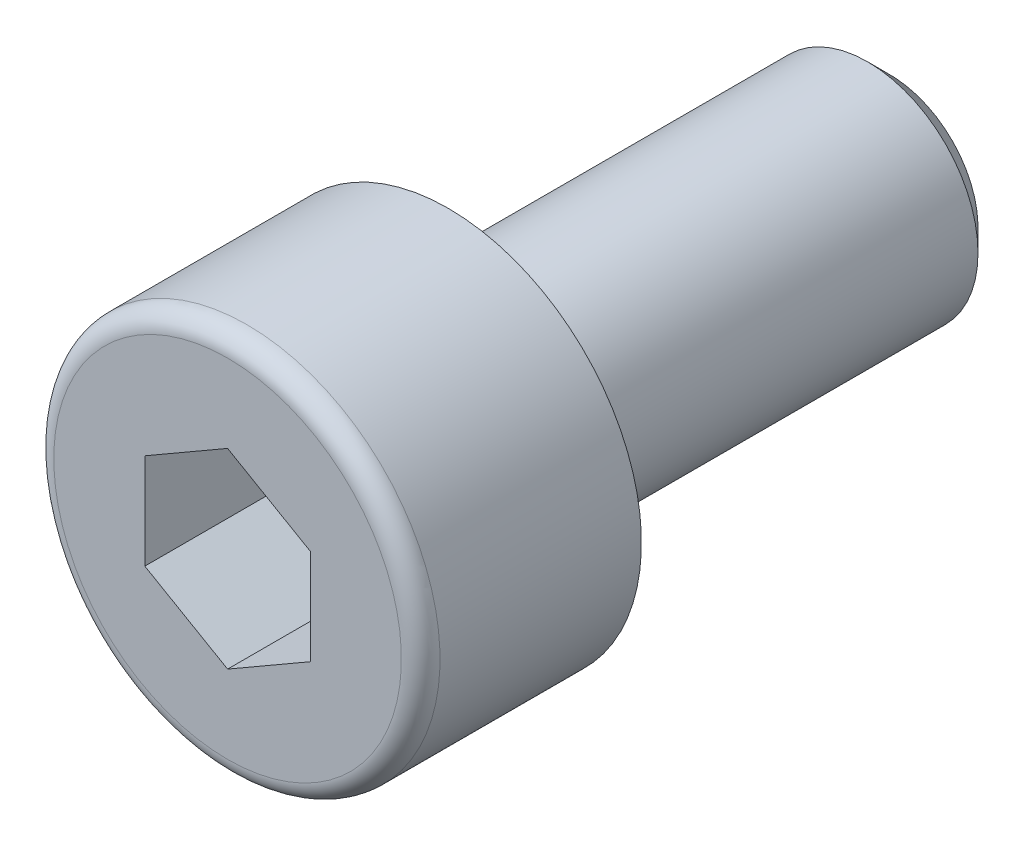
SolidWorks part; units mm, degrees
ref_plane "前视基准面" through (0, 0, 0) normal (0, 0, 1) x (1, 0, 0)
ref_plane "上视基准面" through (0, 0, 0) normal (0, 1, 0) x (1, 0, 0)
ref_plane "右视基准面" through (0, 0, 0) normal (1, 0, 0) x (0, 0, -1)
sketch "草图1" plane through (0, 0, 0) normal (1, 0, 0) x (0, 0, -1)
  line L0 (-4, 0) -> (8, 0) construction
  line L1 (-4, 0) -> (-4, 3.5)
  line L2 (-4, 3.5) -> (0, 3.5)
  line L3 (0, 3.5) -> (0, 2)
  line L4 (0, 2) -> (8, 2)
  line L5 (8, 2) -> (8, 0)
  point P3 (0, 2)
  dimension "A" = 7
  dimension "E" = 4
  dimension "L" = 8
  dimension "(e)" = 8
  dimension "M" = 4
sketch "草图2" plane through (0, 0, 0) normal (0, 0, 1) x (1, 0, 0)
  line L1 (0, 1.7321) -> (-1.5, 0.866)
  line L2 (-1.5, 0.866) -> (-1.5, -0.866)
  line L3 (-1.5, -0.866) -> (0, -1.7321)
  line L4 (0, -1.7321) -> (1.5, -0.866)
  line L5 (1.5, -0.866) -> (1.5, 0.866)
  line L6 (1.5, 0.866) -> (0, 1.7321)
  circle A0 centre (0, 0) radius 1.5 construction
  dimension "B" = 3
sketch "草图3" plane through (0, 0, 0) normal (1, 0, 0) x (0, 0, -1)
  line L0 (-4, 0) -> (-4, 3.5) construction
  line L1 (-4, 3.5) -> (0, 3.5) construction
  line L2 (0, 2) -> (8, 2) construction
  line L3 (0, 3.5) -> (0, 2) construction
  line L4 (-4, 0) -> (8, 0) construction
  line L5 (8, 2) -> (8, 0) construction
  line L6 (-4, 0) -> (-4, 3.5)
  line L7 (-4, 3.5) -> (0, 3.5)
  line L8 (0, 2) -> (8, 2)
  line L9 (0, 3.5) -> (0, 2)
  line L10 (-4, 0) -> (8, 0)
  line L11 (8, 2) -> (8, 0)
revolve "旋转1" add sketch "草图3" angle 360 about L10
cosmetic thread "装饰螺纹线1" parameters "D1"=8, "D2"=3.4
sketch "草图4" plane through (0, 0, 4) normal (0, 0, 1) x (1, 0, 0)
  line L0 (0, 1.7321) -> (-1.5, 0.866) construction
  line L1 (-1.5, 0.866) -> (-1.5, -0.866) construction
  line L2 (-1.5, -0.866) -> (0, -1.7321) construction
  line L3 (0, -1.7321) -> (1.5, -0.866) construction
  line L4 (1.5, -0.866) -> (1.5, 0.866) construction
  line L5 (1.5, 0.866) -> (0, 1.7321) construction
  line L6 (0, 1.7321) -> (-1.5, 0.866)
  line L7 (-1.5, 0.866) -> (-1.5, -0.866)
  line L8 (-1.5, -0.866) -> (0, -1.7321)
  line L9 (0, -1.7321) -> (1.5, -0.866)
  line L10 (1.5, -0.866) -> (1.5, 0.866)
  line L11 (1.5, 0.866) -> (0, 1.7321)
extrude "切除-拉伸1" cut sketch "草图4" against normal blind 2.45
fillet "圆角1" radius 0.35 1 edges at (0, -3.5, 4)
chamfer "倒角1" distance 0.4 angle 45 1 edges at (0, -2, -8)
